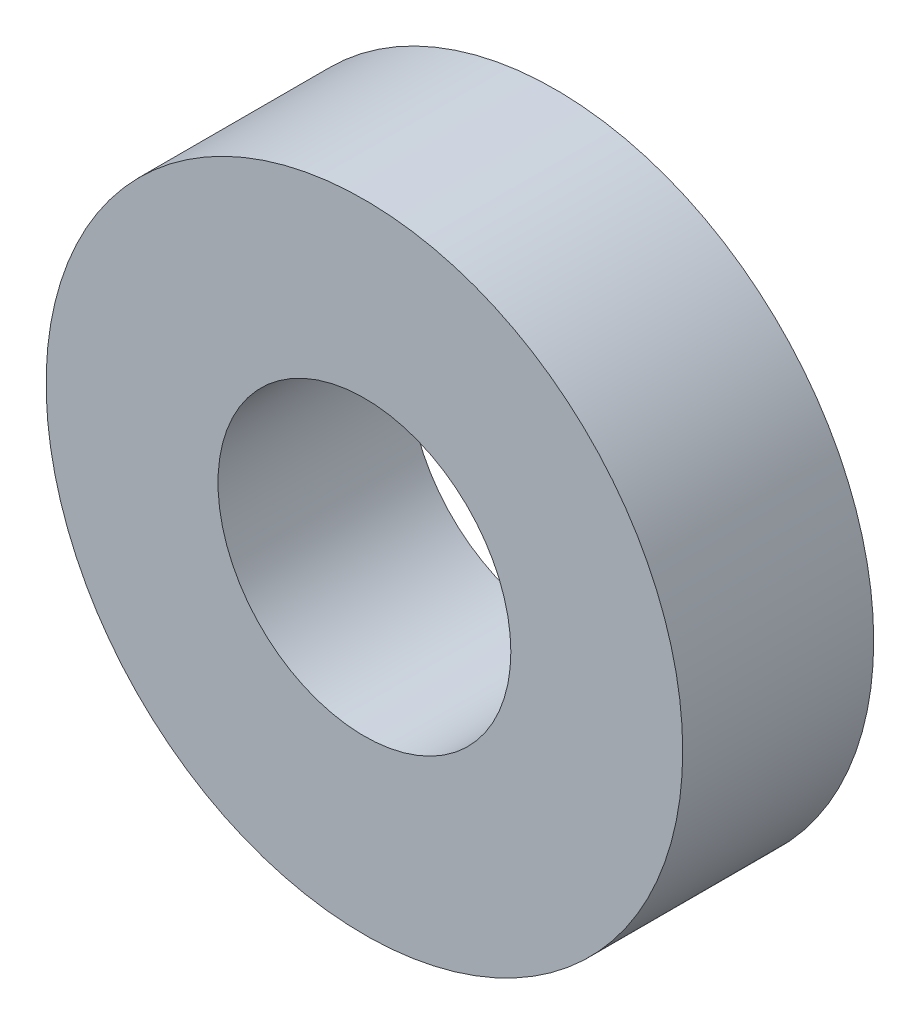
from build123d import *

# Parameters (mm, degrees)
SKETCH1_R           = 5
SKETCH1_R_2         = 2.3
BOSS_EXTRUDE1_DEPTH = 3


with BuildPart() as part:
    # Sketch1 → Boss-Extrude1 (new body)
    with BuildSketch(Plane.XY):
        Circle(SKETCH1_R)
        Circle(SKETCH1_R_2, mode=Mode.SUBTRACT)
    extrude(amount=BOSS_EXTRUDE1_DEPTH)


solid = part.part
